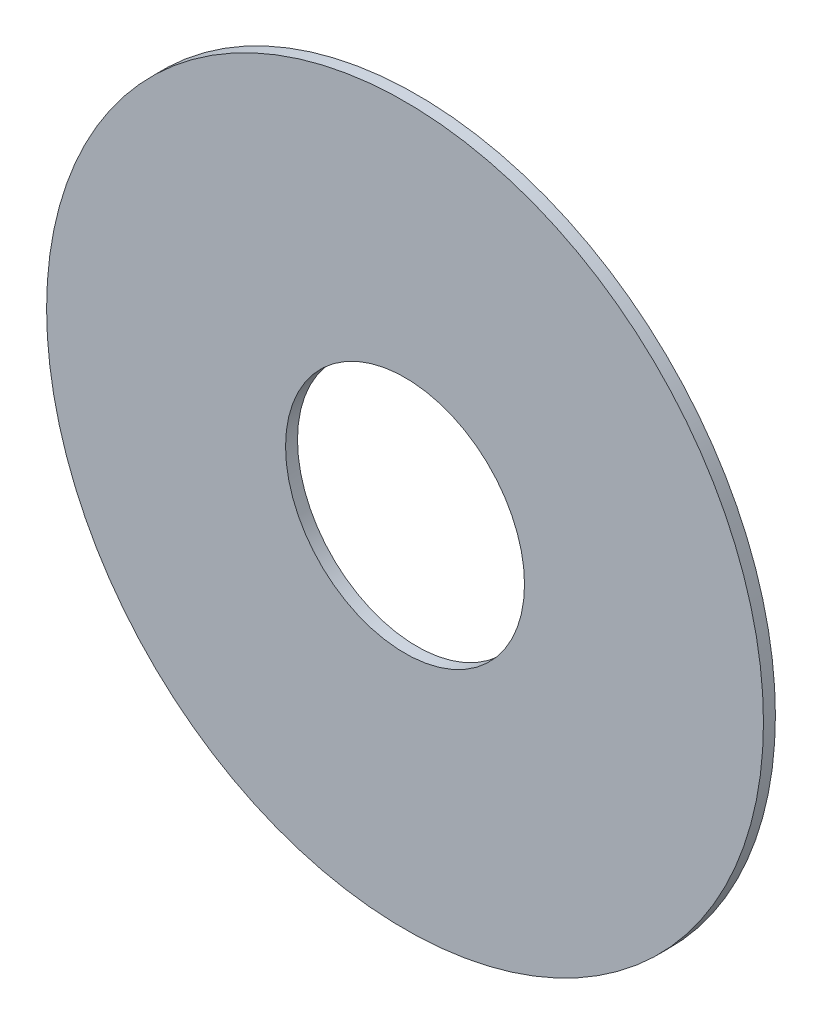
from build123d import *

# Parameters (mm, degrees)
SKETCH1_R           = 30
SKETCH1_R_2         = 10
BOSS_EXTRUDE1_DEPTH = 0.5


with BuildPart() as part:
    # Sketch1 → Boss-Extrude1 (new, symmetric)
    with BuildSketch(Plane.XY):
        Circle(SKETCH1_R)
        Circle(SKETCH1_R_2, mode=Mode.SUBTRACT)
    extrude(amount=BOSS_EXTRUDE1_DEPTH, both=True)


solid = part.part
